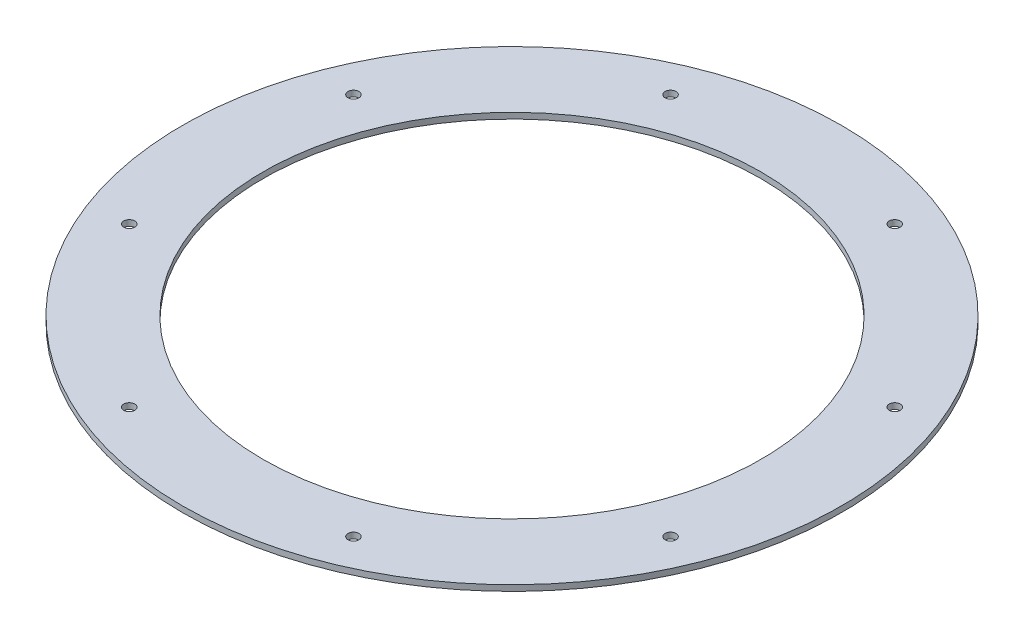
SolidWorks part; units mm, degrees
material "Q235B"
ref_plane "Front Plane" through (0, 0, 0) normal (0, 0, 1) x (1, 0, 0)
ref_plane "Top Plane" through (0, 0, 0) normal (0, 1, 0) x (1, 0, 0)
ref_plane "Right Plane" through (0, 0, 0) normal (1, 0, 0) x (0, 0, -1)
sketch "Sketch1" plane through (0, 0, 0) normal (0, 1, 0) x (1, 0, 0)
  circle A0 centre (0, 0) radius 450
  circle A1 centre (0, 0) radius 340
  dimension "D1" = 900
  dimension "D2" = 680
extrude "Boss-Extrude1" add sketch "Sketch1" along normal mid plane 8
hole_wizard "Ø15.0 (15) Diameter Hole1" positions "Sketch2" profile "Sketch3" hole size "Ø15.0" standard "GB" end condition up to next
sketch "Sketch2" plane through (0, 4, 0) normal (0, 1, 0) x (1, 0, 0)
  line L0 (0, 0) -> (0, 400) construction
  circle A0 centre (0, 0) radius 400 construction
  point P0 (153.0734, 369.5518)
  point P73 (369.5518, 153.0734)
  point P74 (369.5518, -153.0734)
  point P75 (153.0734, -369.5518)
  point P76 (-153.0734, -369.5518)
  point P77 (-369.5518, -153.0734)
  point P78 (-369.5518, 153.0734)
  point P79 (-153.0734, 369.5518)
  dimension "D1" = 800
  dimension "D2" = 8
sketch "Sketch3" plane through (153.0734, 4, -369.5518) normal (1, 0, 0) x (0, 0, 1)
  line L0 (0, 0) -> (0, 8)
  line L1 (0, 8) -> (7.5, 8)
  line L2 (7.5, 8) -> (7.5, 0)
  line L5 (7.5, 0) -> (0, 0)
  line L11 (0, -6.35) -> (0, 107.95) construction
  dimension "通孔孔直径" = 15
  dimension "通孔孔深度" = 8
